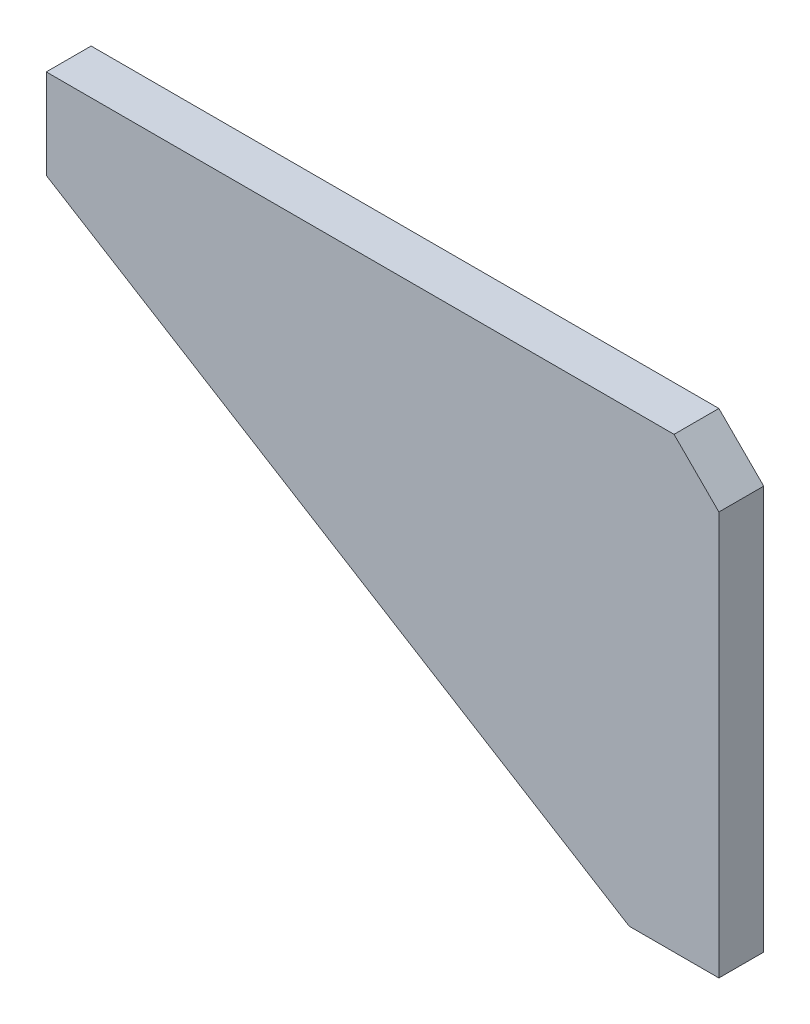
from build123d import *

# Parameters (mm, degrees)
BOSS_EXTRUDE1_DEPTH = 10
CHAMFER1_SIZE       = 10


with BuildPart() as part:
    # Sketch1 → Boss-Extrude1 (new body)
    with BuildSketch(Plane.XY):
        Polygon((0, 0), (-150, 0), (-150, -20), (-20, -100), (0, -100), align=None)
    extrude(amount=-BOSS_EXTRUDE1_DEPTH)

    # Chamfer1
    chamfer1_edges = [part.edges().sort_by_distance(p)[0] for p in [
        (0, 0, -5),
    ]]
    chamfer(chamfer1_edges, length=CHAMFER1_SIZE)


solid = part.part
